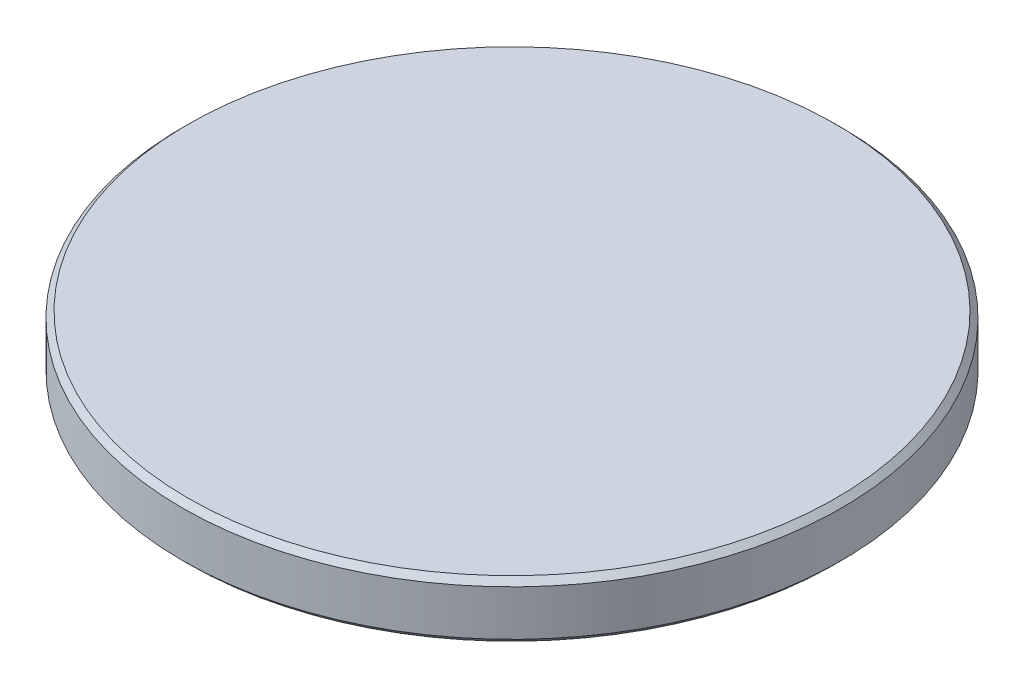
SolidWorks part; units mm, degrees
material "Q235-A"
ref_plane "Front Plane" through (0, 0, 0) normal (0, 0, 1) x (1, 0, 0)
ref_plane "Top Plane" through (0, 0, 0) normal (0, 1, 0) x (1, 0, 0)
ref_plane "Right Plane" through (0, 0, 0) normal (1, 0, 0) x (0, 0, -1)
sketch "Sketch1" plane through (0, 0, 0) normal (0, 1, 0) x (1, 0, 0)
  circle A0 centre (0, 0) radius 58
  dimension "D1" = 116
extrude "Boss-Extrude1" add sketch "Sketch1" along normal blind 10
chamfer "Chamfer1" distance 1 angle 45 2 edges at (0, 0, 58) (0, 10, 58)
